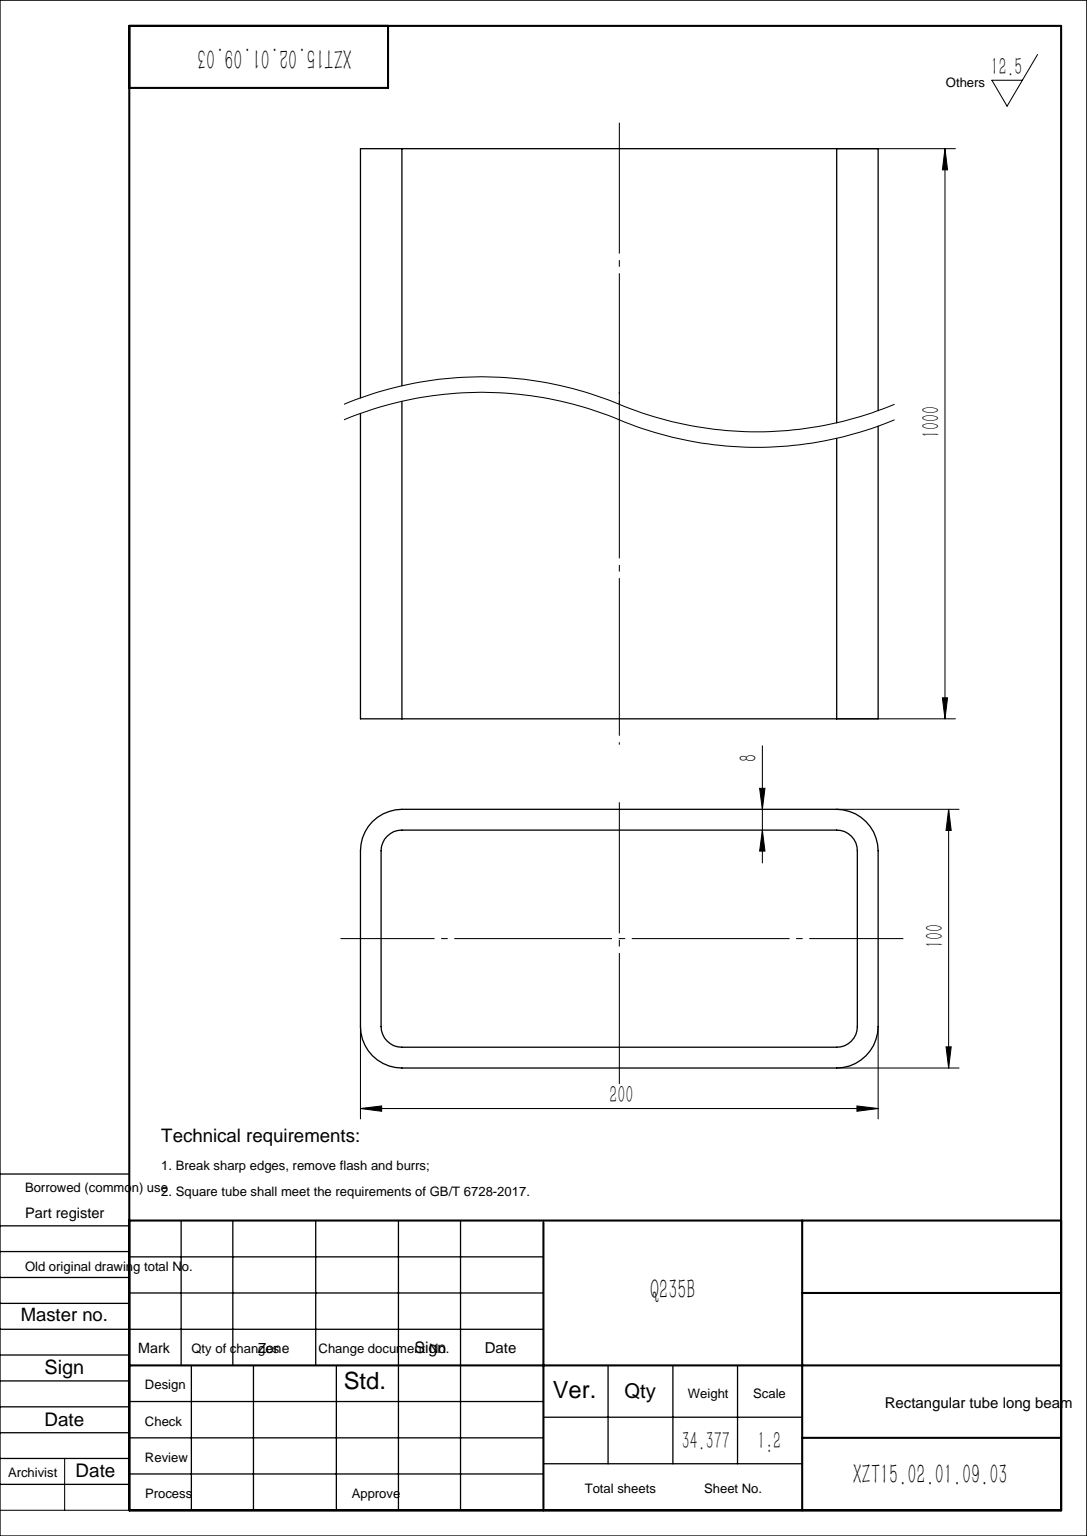
SolidWorks part; units mm, degrees
material "Q235B"
ref_plane "Front Plane" through (0, 0, 0) normal (0, 0, 1) x (1, 0, 0)
ref_plane "Top Plane" through (0, 0, 0) normal (0, 1, 0) x (1, 0, 0)
ref_plane "Right Plane" through (0, 0, 0) normal (1, 0, 0) x (0, 0, -1)
sketch "Sketch1" plane through (0, 0, 0) normal (0, 0, 1) x (1, 0, 0)
  line L0 (0, 0) -> (0, 1000)
  dimension "D1" = 1000
other "GB/T 6728-2002 rectangular hollow section 200X100X8(2)"
ref_plane "Plane1" through (0, 0, 0) normal (0, 1, 0) x (0, 0, 1)
sketch "Sketch12" plane through (0, 0, 0) normal (0, 1, 0) x (0, 0, 1)
  line L0 (-34, -92) -> (34, -92)
  line L1 (-42, -84) -> (-42, 84)
  line L2 (34, 92) -> (-34, 92)
  line L3 (42, 84) -> (42, -84)
  line L4 (-34, -100) -> (34, -100)
  line L5 (-50, -84) -> (-50, 84)
  line L6 (34, 100) -> (-34, 100)
  line L7 (50, 84) -> (50, -84)
  arc A0 (50, 84) -> (34, 100) centre (34, 84) ccw
  arc A1 (34, -100) -> (50, -84) centre (34, -84) ccw
  arc A2 (-50, -84) -> (-34, -100) centre (-34, -84) ccw
  arc A3 (-34, 100) -> (-50, 84) centre (-34, 84) ccw
  arc A4 (-34, 92) -> (-42, 84) centre (-34, 84) ccw
  arc A5 (42, 84) -> (34, 92) centre (34, 84) ccw
  arc A6 (34, -92) -> (42, -84) centre (34, -84) ccw
  arc A7 (-42, -84) -> (-34, -92) centre (-34, -84) ccw
  point P0 (0, 100)
  point P1 (50, 0)
  point P2 (0, -100)
  point P3 (-50, 0)
  point P4 (-50, 100)
  point P5 (50, 100)
  point P6 (50, -100)
  point P7 (-50, -100)
  point P8 (0, 0)
  point P33 (0, 0)
  dimension "D1" = 16
  dimension "Thickness" = 8
  dimension "V_leg" = 200
  dimension "H_leg" = 100
